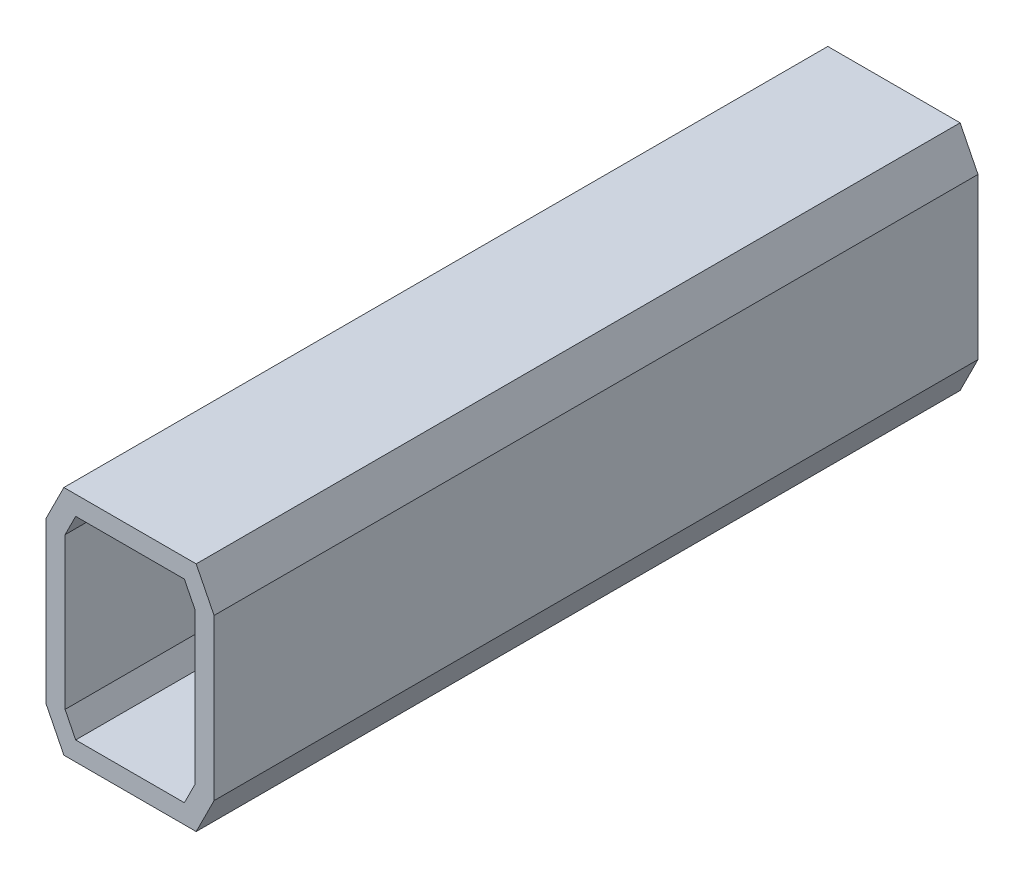
SolidWorks part; units mm, degrees
ref_plane "Front Plane" through (0, 0, 0) normal (0, 0, 1) x (1, 0, 0)
ref_plane "Top Plane" through (0, 0, 0) normal (0, 1, 0) x (1, 0, 0)
ref_plane "Right Plane" through (0, 0, 0) normal (1, 0, 0) x (0, 0, -1)
other "Configuration Table"
sketch "Sketch1" plane through (0, 0, 0) normal (0, 0, 1) x (1, 0, 0)
  line L0 (-17.3197, 136.5) -> (17.3197, 136.5)
  line L3 (17.3197, 136.5) -> (22, 127.1393)
  line L4 (22, 127.1393) -> (22, 85.1607)
  line L5 (22, 85.1607) -> (17.3197, 75.8)
  line L6 (17.3197, 75.8) -> (-17.3197, 75.8)
  line L7 (-17.3197, 75.8) -> (-22, 85.1607)
  line L8 (-22, 85.1607) -> (-22, 127.1393)
  line L9 (-22, 127.1393) -> (-17.3197, 136.5)
  line L10 (-14.2295, 131.5) -> (14.2295, 131.5)
  line L11 (14.2295, 131.5) -> (17, 125.959)
  line L12 (17, 125.959) -> (17, 86.341)
  line L13 (17, 86.341) -> (14.2295, 80.8)
  line L14 (14.2295, 80.8) -> (-14.2295, 80.8)
  line L15 (-14.2295, 80.8) -> (-17, 86.341)
  line L16 (-17, 86.341) -> (-17, 125.959)
  line L17 (-17, 125.959) -> (-14.2295, 131.5)
  dimension "D1" = 5
extrude "Boss-Extrude1" add sketch "Sketch1" along normal blind 200
